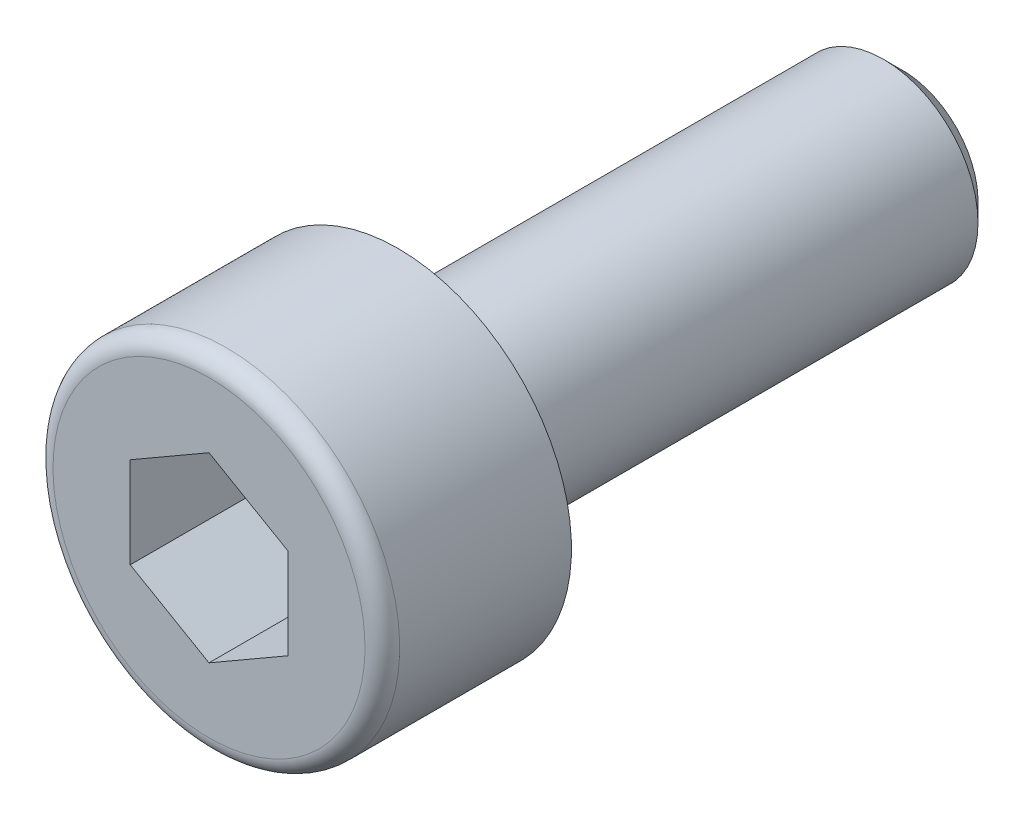
SolidWorks part; units mm, degrees
ref_plane "前视基准面" through (0, 0, 0) normal (0, 0, 1) x (1, 0, 0)
ref_plane "上视基准面" through (0, 0, 0) normal (0, 1, 0) x (1, 0, 0)
ref_plane "右视基准面" through (0, 0, 0) normal (1, 0, 0) x (0, 0, -1)
sketch "草图1" plane through (0, 0, 0) normal (1, 0, 0) x (0, 0, -1)
  line L0 (-3, 0) -> (8, 0) construction
  line L1 (-3, 0) -> (-3, 2.75)
  line L2 (-3, 2.75) -> (0, 2.75)
  line L3 (0, 2.75) -> (0, 1.5)
  line L4 (0, 1.5) -> (8, 1.5)
  line L5 (8, 1.5) -> (8, 0)
  point P3 (0, 1.5)
  dimension "A" = 5.5
  dimension "E" = 3
  dimension "L" = 8
  dimension "(e)" = 8
  dimension "M" = 3
sketch "草图2" plane through (0, 0, 0) normal (0, 0, 1) x (1, 0, 0)
  line L1 (0, 1.4434) -> (-1.25, 0.7217)
  line L2 (-1.25, 0.7217) -> (-1.25, -0.7217)
  line L3 (-1.25, -0.7217) -> (0, -1.4434)
  line L4 (0, -1.4434) -> (1.25, -0.7217)
  line L5 (1.25, -0.7217) -> (1.25, 0.7217)
  line L6 (1.25, 0.7217) -> (0, 1.4434)
  circle A0 centre (0, 0) radius 1.25 construction
  dimension "B" = 2.5
sketch "草图3" plane through (0, 0, 0) normal (1, 0, 0) x (0, 0, -1)
  line L0 (-3, 0) -> (-3, 2.75) construction
  line L1 (-3, 2.75) -> (0, 2.75) construction
  line L2 (0, 1.5) -> (8, 1.5) construction
  line L3 (0, 2.75) -> (0, 1.5) construction
  line L4 (-3, 0) -> (8, 0) construction
  line L5 (8, 1.5) -> (8, 0) construction
  line L6 (-3, 0) -> (-3, 2.75)
  line L7 (-3, 2.75) -> (0, 2.75)
  line L8 (0, 1.5) -> (8, 1.5)
  line L9 (0, 2.75) -> (0, 1.5)
  line L10 (-3, 0) -> (8, 0)
  line L11 (8, 1.5) -> (8, 0)
revolve "旋转1" add sketch "草图3" angle 360 about L10
cosmetic thread "装饰螺纹线1" parameters "D1"=8, "D2"=2.55
sketch "草图4" plane through (0, 0, 3) normal (0, 0, 1) x (1, 0, 0)
  line L0 (0, 1.4434) -> (-1.25, 0.7217) construction
  line L1 (-1.25, 0.7217) -> (-1.25, -0.7217) construction
  line L2 (-1.25, -0.7217) -> (0, -1.4434) construction
  line L3 (0, -1.4434) -> (1.25, -0.7217) construction
  line L4 (1.25, -0.7217) -> (1.25, 0.7217) construction
  line L5 (1.25, 0.7217) -> (0, 1.4434) construction
  line L6 (0, 1.4434) -> (-1.25, 0.7217)
  line L7 (-1.25, 0.7217) -> (-1.25, -0.7217)
  line L8 (-1.25, -0.7217) -> (0, -1.4434)
  line L9 (0, -1.4434) -> (1.25, -0.7217)
  line L10 (1.25, -0.7217) -> (1.25, 0.7217)
  line L11 (1.25, 0.7217) -> (0, 1.4434)
extrude "切除-拉伸1" cut sketch "草图4" against normal blind 1.925
fillet "圆角1" radius 0.275 1 edges at (0, -2.75, 3)
chamfer "倒角1" distance 0.3 angle 45 1 edges at (0, -1.5, -8)
